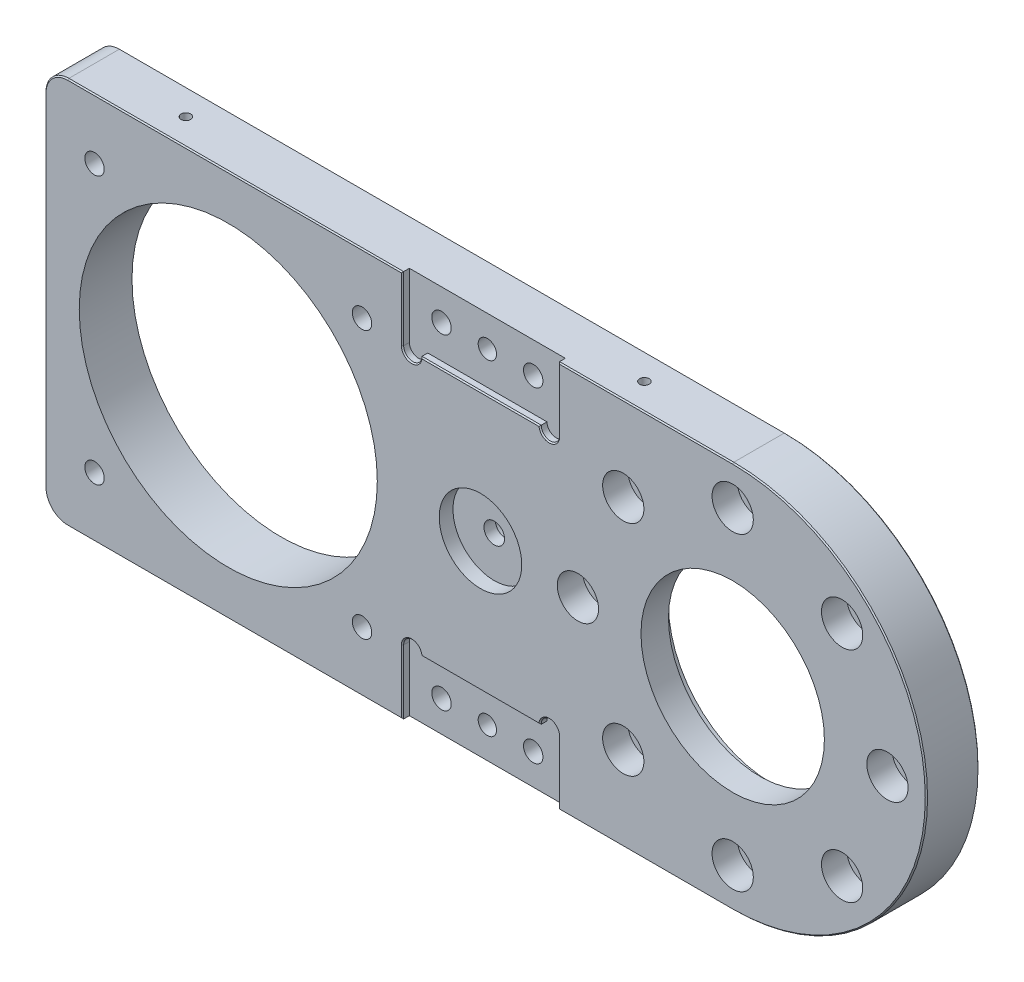
from build123d import *

# Parameters (mm, degrees)
BOSS_EXTRUDE1_DEPTH                                = 23
FILLET1_R                                          = 10
HOLE_SIZE_BASED_ON_SOCKET_HEAD_CAP_SCR_D           = 11
HOLE_SIZE_BASED_ON_SOCKET_HEAD_CAP_SCR_CBORE_D     = 18
HOLE_SIZE_BASED_ON_SOCKET_HEAD_CAP_SCR_CBORE_DEPTH = 11
CIRPATTERN1_COUNT                                  = 8
SKETCH8_R                                          = 65
CUT_EXTRUDE1_DEPTH                                 = 23
SKETCH9_R                                          = 18
CUT_EXTRUDE2_DEPTH                                 = 6
HOLE_WIZARD_3_D                                    = 9
HOLE_WIZARD_3_CBORE_D                              = 15
HOLE_WIZARD_3_CBORE_DEPTH                          = 12
SKETCH13_R                                         = 40
CUT_EXTRUDE3_DEPTH                                 = 23
SKETCH14_R                                         = 57.5
CUT_EXTRUDE4_DEPTH                                 = 6
M10_TAPPED_HOLE3_D                                 = 8.5
M5_TAPPED_HOLE1_AT_2_COUNT                         = 2
M5_TAPPED_HOLE1_AT_2_PITCH                         = 200
M10_TAPPED_HOLE5_D                                 = 8.5
CHAMFER1_SIZE                                      = 0.5
SKETCH23_R                                         = 45
CUT_EXTRUDE5_DEPTH                                 = 5
SKETCH24_W                                         = 68
SKETCH24_H                                         = 28
CUT_EXTRUDE6_DEPTH                                 = 3
SKETCH25_R                                         = 4
CUT_EXTRUDE7_DEPTH                                 = 3
CHAMFER2_SIZE                                      = 0.5


with BuildPart() as part:
    # Sketch1 → Boss-Extrude1 (new body)
    with BuildSketch(Plane.XY):
        with BuildLine():
            Line((0, 0), (300, 0))
            ThreePointArc((300, 0), (384.5, 84.5), (300, 169))
            Line((300, 169), (0, 169))
            Line((0, 169), (0, 0))
        make_face()
    extrude(amount=BOSS_EXTRUDE1_DEPTH)

    # Fillet1
    fillet1_edges = [part.edges().sort_by_distance(p)[0] for p in [
        (0, 169, 11.5),
        (0, 0, 11.5),
    ]]
    fillet(fillet1_edges, radius=FILLET1_R)

    # Hole size (% based on socket head cap screw type)3 (through all)
    with Locations(Plane.XY.offset(23)):
        with Locations((300, 17)):
            hole_size_based_on_socket_head_cap_scr = CounterBoreHole(HOLE_SIZE_BASED_ON_SOCKET_HEAD_CAP_SCR_D / 2, HOLE_SIZE_BASED_ON_SOCKET_HEAD_CAP_SCR_CBORE_D / 2, HOLE_SIZE_BASED_ON_SOCKET_HEAD_CAP_SCR_CBORE_DEPTH)

    # CirPattern1: Hole size (% based on socket head cap screw type)3 ×8 about axis
    cirpattern1_axis = Axis((300, 84.5, 0), (0, 0, 1))
    for i in range(1, CIRPATTERN1_COUNT):
        add(hole_size_based_on_socket_head_cap_scr.rotate(cirpattern1_axis, i * 360 / CIRPATTERN1_COUNT), mode=Mode.SUBTRACT)

    # Sketch8 → Cut-Extrude1 (cut)
    with BuildSketch(Plane.XY.offset(23)):
        with Locations((80, 84.5)):
            Circle(SKETCH8_R)
    extrude(amount=-CUT_EXTRUDE1_DEPTH, mode=Mode.SUBTRACT)

    # Sketch9 → Cut-Extrude2 (cut)
    with BuildSketch(Plane.XY.offset(23)):
        with Locations((190, 84.5)):
            Circle(SKETCH9_R)
    extrude(amount=-CUT_EXTRUDE2_DEPTH, mode=Mode.SUBTRACT)

    # Hole Wizard 3 (through all)
    with Locations(Plane(origin=(0, 0, 0), x_dir=(-1, 0, 0), z_dir=(0, 0, -1))):
        with Locations((-190, 84.5)):
            CounterBoreHole(HOLE_WIZARD_3_D / 2, HOLE_WIZARD_3_CBORE_D / 2, HOLE_WIZARD_3_CBORE_DEPTH)

    # Sketch13 → Cut-Extrude3 (cut)
    with BuildSketch(Plane(origin=(0, 0, 0), x_dir=(-1, 0, 0), z_dir=(0, 0, -1))):
        with Locations((-300, 84.5)):
            Circle(SKETCH13_R)
    extrude(amount=-CUT_EXTRUDE3_DEPTH, mode=Mode.SUBTRACT)

    # Sketch14 → Cut-Extrude4 (cut)
    with BuildSketch(Plane(origin=(0, 0, 0), x_dir=(-1, 0, 0), z_dir=(0, 0, -1))):
        with Locations((-300, 84.5)):
            Circle(SKETCH14_R)
    extrude(amount=-CUT_EXTRUDE4_DEPTH, mode=Mode.SUBTRACT)

    # M10 Tapped Hole3 (through all)
    with Locations(Plane(origin=(0, 0, 0), x_dir=(-1, 0, 0), z_dir=(0, 0, -1))):
        with Locations((-21.663690552, 26.163690552), (-138.336309448, 26.163690552), (-21.663690552, 142.836309448), (-138.336309448, 142.836309448), (-80, 84.5)):
            Hole(M10_TAPPED_HOLE3_D / 2)

    # Sketch18 → M5 Tapped Hole1 (revolve, cut)
    with BuildSketch(Plane(origin=(50, 169, 11.5), x_dir=(0, 0, 1), z_dir=(1, 0, 0))):
        Polygon((0, 0), (0, 13.6618073), (2.1, 12.4), (2.1, 0), align=None)
    m5_tapped_hole1 = revolve(axis=Axis((50, 175.35, 11.5), (0, -1, 0)), mode=Mode.SUBTRACT)

    # M5 Tapped Hole1 at 2: M5 Tapped Hole1 ×2
    with Locations(*[(i * M5_TAPPED_HOLE1_AT_2_PITCH, 0, 0) for i in range(1, M5_TAPPED_HOLE1_AT_2_COUNT)]):
        add(m5_tapped_hole1, mode=Mode.SUBTRACT)

    # Mirror1: M5 Tapped Hole1 across plane
    add(m5_tapped_hole1.mirror(Plane.ZX.offset(84.5)), mode=Mode.SUBTRACT)

    # Mirror1 copy 1 sketch → Mirror1 copy 1 (revolve, cut)
    with BuildSketch(Plane(origin=(250, 0, 11.5), x_dir=(0, 0, 1), z_dir=(1, 0, 0))):
        Polygon((0, 0), (0, -13.6618073), (2.1, -12.4), (2.1, 0), align=None)
    revolve(axis=Axis((250, -6.35, 11.5), (0, -1, 0)), mode=Mode.SUBTRACT)

    # M10 Tapped Hole5 (through all)
    with Locations(Plane.XY.offset(23)):
        with Locations((170, 155.5), (210, 155.5)):
            m10_tapped_hole5 = Hole(M10_TAPPED_HOLE5_D / 2)

    # Mirror2: M10 Tapped Hole5 across plane
    add(m10_tapped_hole5.mirror(Plane.ZX.offset(84.5)), mode=Mode.SUBTRACT)

    # Chamfer1
    chamfer1_edges = [part.edges().sort_by_distance(p)[0] for p in [
        (155, 0, 0),
        (0, 84.5, 0),
        (2.928932188, 166.071067812, 0),
        (2.928932188, 2.928932188, 0),
        (155, 169, 0),
        (384.5, 84.5, 0),
    ]]
    chamfer(chamfer1_edges, length=CHAMFER1_SIZE)

    # Sketch23 → Cut-Extrude5 (cut)
    with BuildSketch(Plane(origin=(0, 0, 6), x_dir=(-1, 0, 0), z_dir=(0, 0, -1))):
        with Locations((-300, 84.5)):
            Circle(SKETCH23_R)
    extrude(amount=-CUT_EXTRUDE5_DEPTH, mode=Mode.SUBTRACT)

    # Sketch24 → Cut-Extrude6 (cut)
    with BuildSketch(Plane.XY.offset(23)):
        with Locations((190, 155)):
            Rectangle(SKETCH24_W, SKETCH24_H)
    cut_extrude6 = extrude(amount=-CUT_EXTRUDE6_DEPTH, mode=Mode.SUBTRACT)

    # Mirror3: Cut-Extrude6 across plane
    add(cut_extrude6.mirror(Plane.ZX.offset(84.5)), mode=Mode.SUBTRACT)

    # Sketch25 → Cut-Extrude7 (cut)
    with BuildSketch(Plane.XY.offset(23)):
        with Locations((160, 141)):
            Circle(SKETCH25_R)
        with Locations((220, 141)):
            Circle(SKETCH25_R)
    cut_extrude7 = extrude(amount=-CUT_EXTRUDE7_DEPTH, mode=Mode.SUBTRACT)

    # Mirror4: Cut-Extrude7 across plane
    add(cut_extrude7.mirror(Plane.ZX.offset(84.5)), mode=Mode.SUBTRACT)

    # Sketch28 → Size mm, blind dowel hole 1 (revolve, cut)
    with BuildSketch(Plane(origin=(190, 13.5, 20), x_dir=(0, -1, 0), z_dir=(1, 0, 0))):
        Polygon((0, 0), (0, 17.403442476), (4, 15), (4, 0), align=None)
    size_mm_blind_dowel_hole_1 = revolve(axis=Axis((190, 13.5, 26.35), (0, 0, -1)), mode=Mode.SUBTRACT)

    # Mirror5: Size mm, blind dowel hole 1 across plane
    add(size_mm_blind_dowel_hole_1.mirror(Plane.ZX.offset(84.5)), mode=Mode.SUBTRACT)

    # Chamfer2
    chamfer2_edges = [part.edges().sort_by_distance(p)[0] for p in [
        (384.5, 84.5, 23),
        (262, 169, 23),
        (83, 0, 23),
        (0, 84.5, 23),
        (2.928932188, 166.071067812, 23),
        (2.928932188, 2.928932188, 23),
        (83, 169, 23),
        (156, 155, 23),
        (224, 155, 23),
        (262, 0, 23),
        (156, 14, 23),
        (224, 14, 23),
        (190, 141, 23),
        (160, 137, 23),
        (220, 137, 23),
        (190, 28, 23),
        (160, 32, 23),
        (220, 32, 23),
    ]]
    chamfer(chamfer2_edges, length=CHAMFER2_SIZE)


solid = part.part
